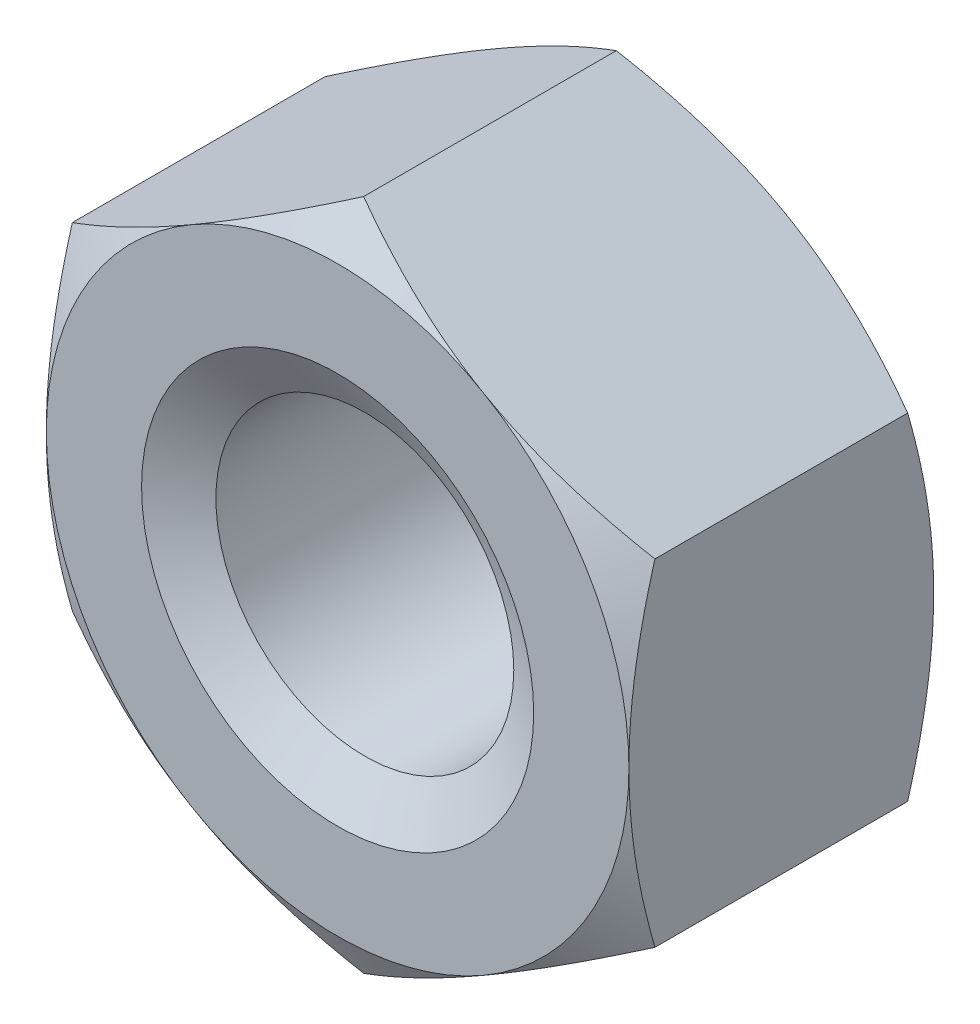
SolidWorks part; units mm, degrees
ref_plane "前视基准面" through (0, 0, 0) normal (0, 0, 1) x (1, 0, 0)
ref_plane "上视基准面" through (0, 0, 0) normal (0, 1, 0) x (1, 0, 0)
ref_plane "右视基准面" through (0, 0, 0) normal (1, 0, 0) x (0, 0, -1)
sketch "草图1" plane through (0, 0, 0) normal (1, 0, 0) x (0, 0, -1)
  line L0 (0, 7.19) -> (0, -7.19) construction
  line L1 (0, 0) -> (6.8, 0) construction
  line L2 (0, 0) -> (0, 7.19)
  line L3 (0, 7.19) -> (6.8, 7.19)
  line L4 (6.8, 7.19) -> (6.8, 0)
  line L5 (0, 4) -> (6.8, 4)
  line L6 (0, 3.3234) -> (6.8, 3.3234)
  line L7 (6.2, 7.19) -> (6.2, 0)
  line L8 (0, 6.5) -> (0.3984, 7.19)
  line L9 (0, 4) -> (0.3906, 3.3234)
  line L10 (0, -4) -> (0.3906, -3.3234)
  line L11 (6.2, 5.8) -> (6.8, 5.8)
  point P5 (1.6, 0)
  point P10 (5.55, 0)
  point P22 (0, 8.75)
  dimension "e" = 14.38
  dimension "m" = 6.8
  dimension "mw" = 5.2
  dimension "D" = 8
  dimension "P" = 1.25
  dimension "D81" = 6.6469
  dimension "c" = 0.6
  dimension "β" = 30
  dimension "s" = 13
  dimension "θ" = 120
  dimension "dw" = 11.6
  dimension "da" = 8.75
sketch "草图2" plane through (0, 0, 0) normal (0, 0, 1) x (1, 0, 0)
  line L1 (0, 7.5056) -> (-6.5, 3.7528)
  line L2 (-6.5, 3.7528) -> (-6.5, -3.7528)
  line L3 (-6.5, -3.7528) -> (0, -7.5056)
  line L4 (0, -7.5056) -> (6.5, -3.7528)
  line L5 (6.5, -3.7528) -> (6.5, 3.7528)
  line L6 (6.5, 3.7528) -> (0, 7.5056)
  circle A0 centre (0, 0) radius 6.5 construction
  circle A1 centre (0, 0) radius 3.3234
  dimension "D1" = 13
sketch "草图3" plane through (0, 0, 0) normal (0, 0, 1) x (1, 0, 0)
  line L0 (0, 7.5056) -> (-6.5, 3.7528) construction
  line L1 (6.5, 3.7528) -> (0, 7.5056) construction
  line L2 (6.5, -3.7528) -> (6.5, 3.7528) construction
  line L3 (0, -7.5056) -> (6.5, -3.7528) construction
  line L4 (-6.5, -3.7528) -> (0, -7.5056) construction
  line L5 (-6.5, 3.7528) -> (-6.5, -3.7528) construction
  line L6 (0, 7.5056) -> (-6.5, 3.7528)
  line L7 (6.5, 3.7528) -> (0, 7.5056)
  line L8 (6.5, -3.7528) -> (6.5, 3.7528)
  line L9 (0, -7.5056) -> (6.5, -3.7528)
  line L10 (-6.5, -3.7528) -> (0, -7.5056)
  line L11 (-6.5, 3.7528) -> (-6.5, -3.7528)
  circle A0 centre (0, 0) radius 3.3234 construction
  circle A1 centre (0, 0) radius 3.3234
extrude "凸台-拉伸1" add sketch "草图3" against normal up to vertex (6.8 mm away) up to point (0, 0, -6.8)
cosmetic thread "装饰螺纹线1" parameters "D2"=8
sketch "草图4" plane through (0, 0, 0) normal (1, 0, 0) x (0, 0, -1)
  line L1 (0, 4.375) -> (0.6071, 3.3234)
  line L2 (0, 0) -> (6.8, 0) construction
  line L3 (0, 0) -> (6.8, 0) construction
  line L4 (3.4, 0) -> (3.4, 7.19) construction
  line L5 (0, 7.19) -> (6.8, 7.19) construction
  line L6 (0.6071, 3.3234) -> (0.6071, 0)
  line L7 (0.6071, 0) -> (0, 0)
  line L8 (0, 0) -> (0, 4.375)
  line L9 (6.8, 0) -> (6.8, 4.375)
  line L10 (6.1929, 0) -> (6.8, 0)
  line L11 (6.1929, 3.3234) -> (6.1929, 0)
  line L12 (6.8, 4.375) -> (6.1929, 3.3234)
  line L16 (0, 4) -> (0.3906, 3.3234) construction
  line L17 (0, 3.3234) -> (6.8, 3.3234) construction
  dimension "D1" = 8.75
revolve "切除-旋转1" cut sketch "草图4" angle 360 mid plane about L3
sketch "草图5" plane through (0, 0, 0) normal (0, 0, 1) x (1, 0, 0)
  circle A0 centre (0, 0) radius 6.5
  circle A1 centre (0, 0) radius 10.785
  circle A2 centre (0, 0) radius 6.5 construction
  dimension "D1" = 21.57
extrude "切除-拉伸1" cut sketch "草图5" against normal blind 1.36 draft 60
sketch "草图7" plane through (0, 0, -6.8) normal (0, 0, -1) x (-1, 0, 0)
  circle A1 centre (0, 0) radius 10.785
  circle A2 centre (0, 0) radius 10.785
  circle A3 centre (0, 0) radius 6.5
  circle A4 centre (0, 0) radius 6.5
  dimension "D1" = 0
  dimension "D2" = 0
extrude "切除-拉伸2" cut sketch "草图7" against normal blind 1.36 draft 60
sketch "草图6" [suppressed] plane through (0, 0, 0) normal (1, 0, 0) x (0, 0, -1)
  line L0 (51, 44.1) -> (50, 44.1)
  line L1 (50, 44.1) -> (50, 54.8483)
  line L2 (50, 54.8483) -> (51, 54.8483)
  line L3 (51, 54.8483) -> (51, 44.1)
  line L4 (0, 0) -> (51, 0) construction
  line L5 (0, 0) -> (51, 0) construction
  line L6 (46.7575, 54.8483) -> (4.2425, 54.8483) construction
revolve "切除-旋转2" [suppressed] cut sketch "草图6" angle 360 mid plane about L5
